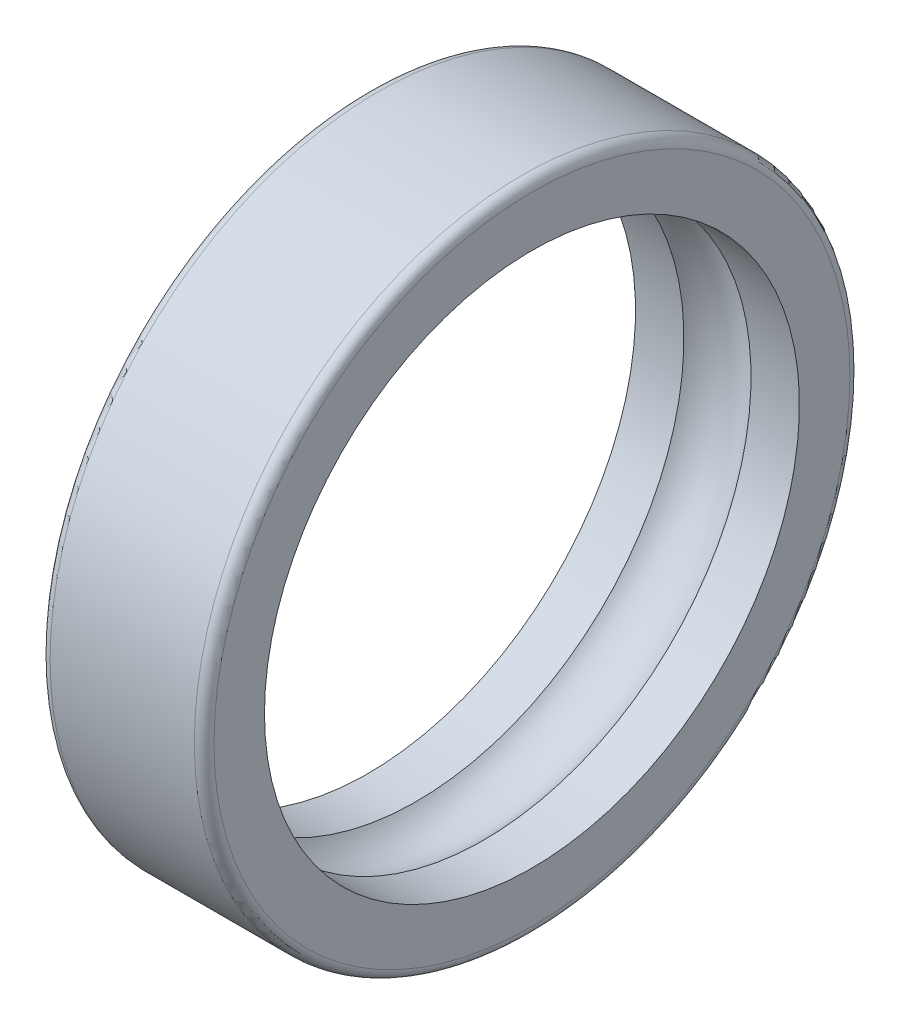
from build123d import *

# Parameters (mm, degrees)
FILLET1_R = 1.5


with BuildPart() as part:
    # Sketch1 → Revolve1 (revolve)
    with BuildSketch(Plane.XY, mode=Mode.PRIVATE) as revolve1_sk:
        with BuildLine():
            Line((5.120546846, 40.8), (12.5, 40.8))
            Line((12.5, 40.8), (12.5, 50))
            Line((12.5, 50), (-12.5, 50))
            Line((-12.5, 50), (-12.5, 40.8))
            Line((-12.5, 40.8), (-5.120546846, 40.8))
            ThreePointArc((-5.120546846, 40.8), (0, 43.1), (5.120546846, 40.8))
        make_face()
    revolve(revolve1_sk.sketch.rotate(Axis((-5.850943074, 0, 0), (1, 0, 0)), 90), axis=Axis((-5.850943074, 0, 0), (1, 0, 0)))

    # Fillet1
    fillet1_edges = [part.edges().sort_by_distance(p)[0] for p in [
        (-12.5, 0, -50),
        (12.5, 0, -50),
    ]]
    fillet(fillet1_edges, radius=FILLET1_R)


solid = part.part
